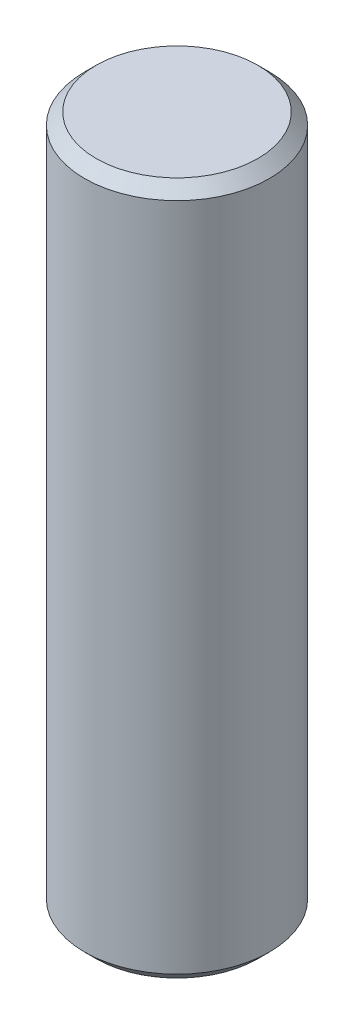
SolidWorks part; units mm, degrees
ref_plane "Front Plane" through (0, 0, 0) normal (0, 0, 1) x (1, 0, 0)
ref_plane "Top Plane" through (0, 0, 0) normal (0, 1, 0) x (1, 0, 0)
ref_plane "Right Plane" through (0, 0, 0) normal (1, 0, 0) x (0, 0, -1)
other "Configuration Table"
sketch "Sketch1" plane through (0, 0, 0) normal (0, 1, 0) x (1, 0, 0)
  circle A0 centre (0, 0) radius 4
  dimension "D1" = 8
extrude "Boss-Extrude1" add sketch "Sketch1" along normal mid plane 30 contours A0
chamfer "Chamfer1" distance 0.5 angle 45 2 edges at (0, -15, 4) (0, 15, 4)
